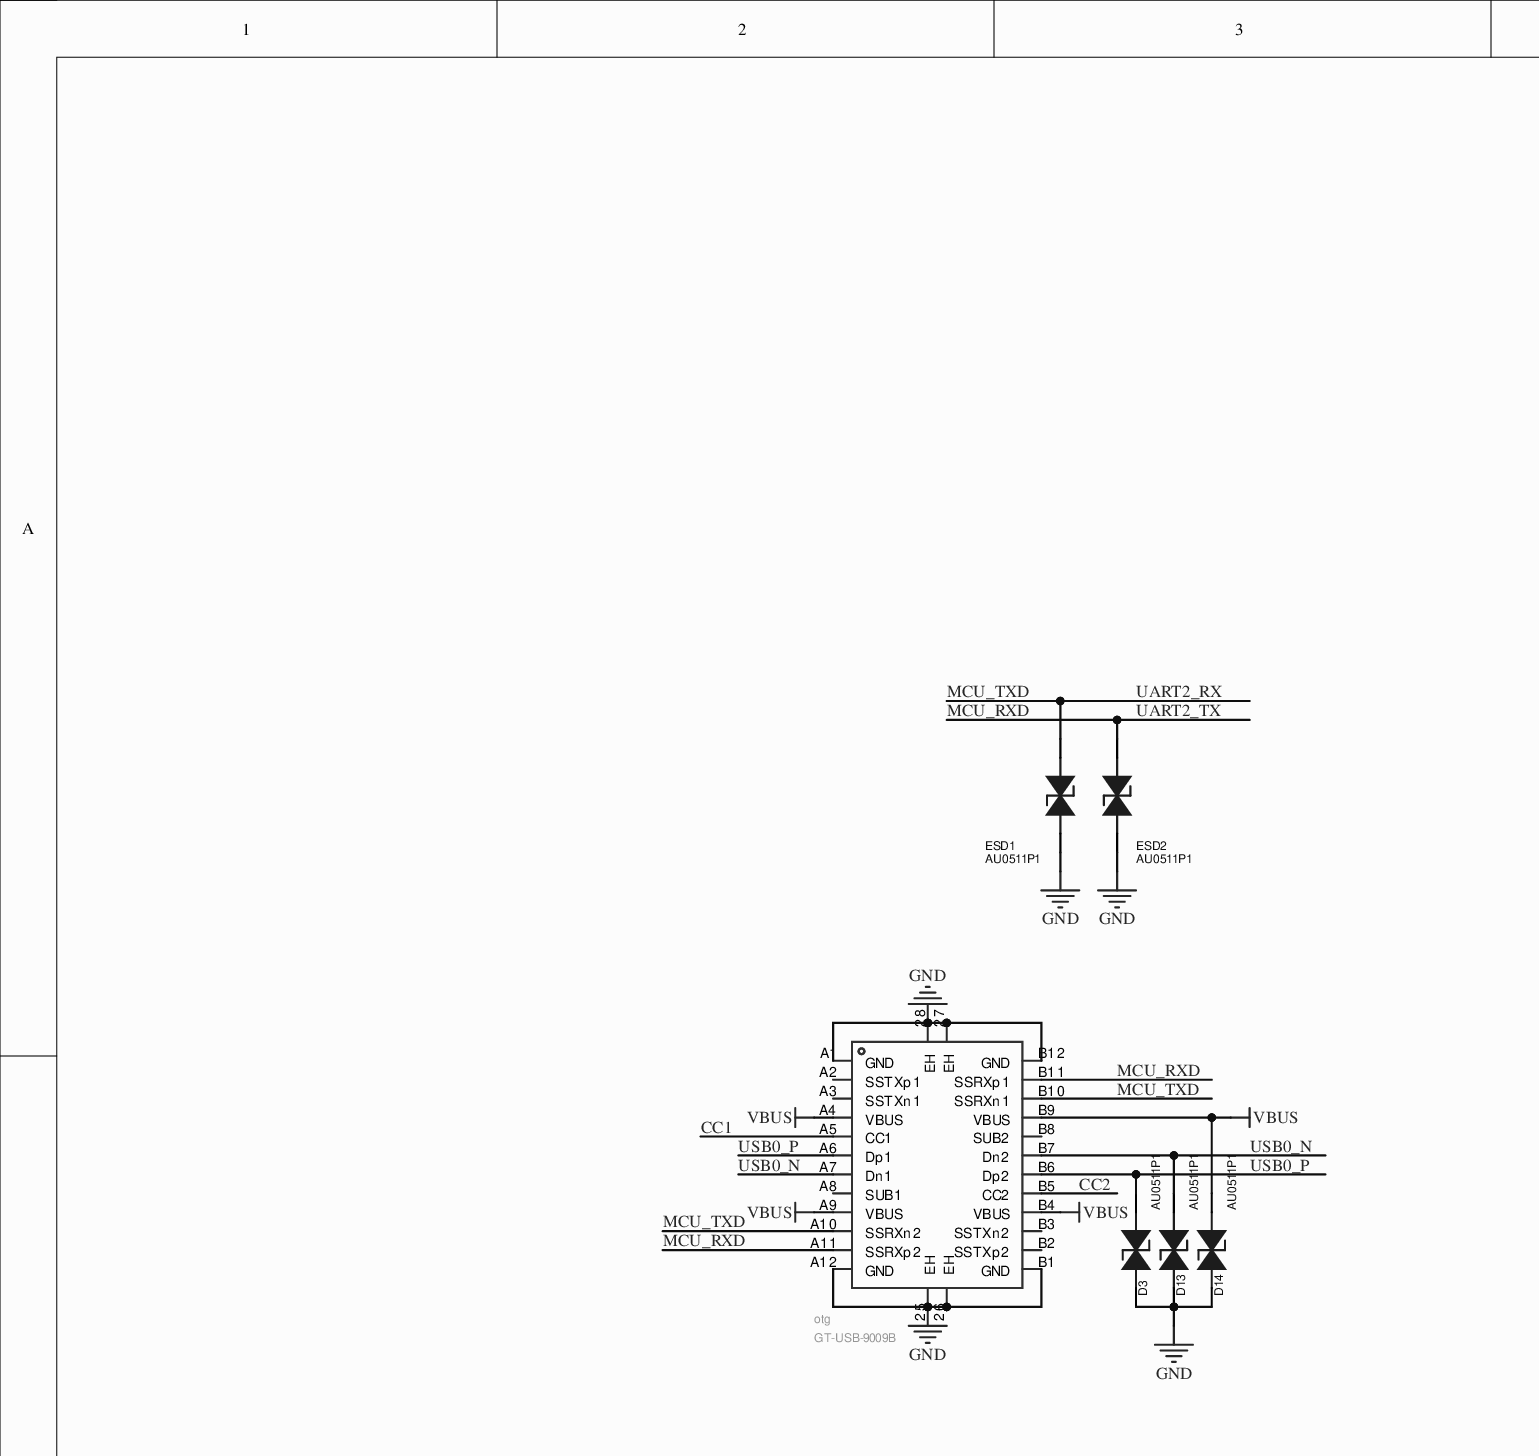
[diagram p0: MISC105407.SchDoc, top column 1 of 4]
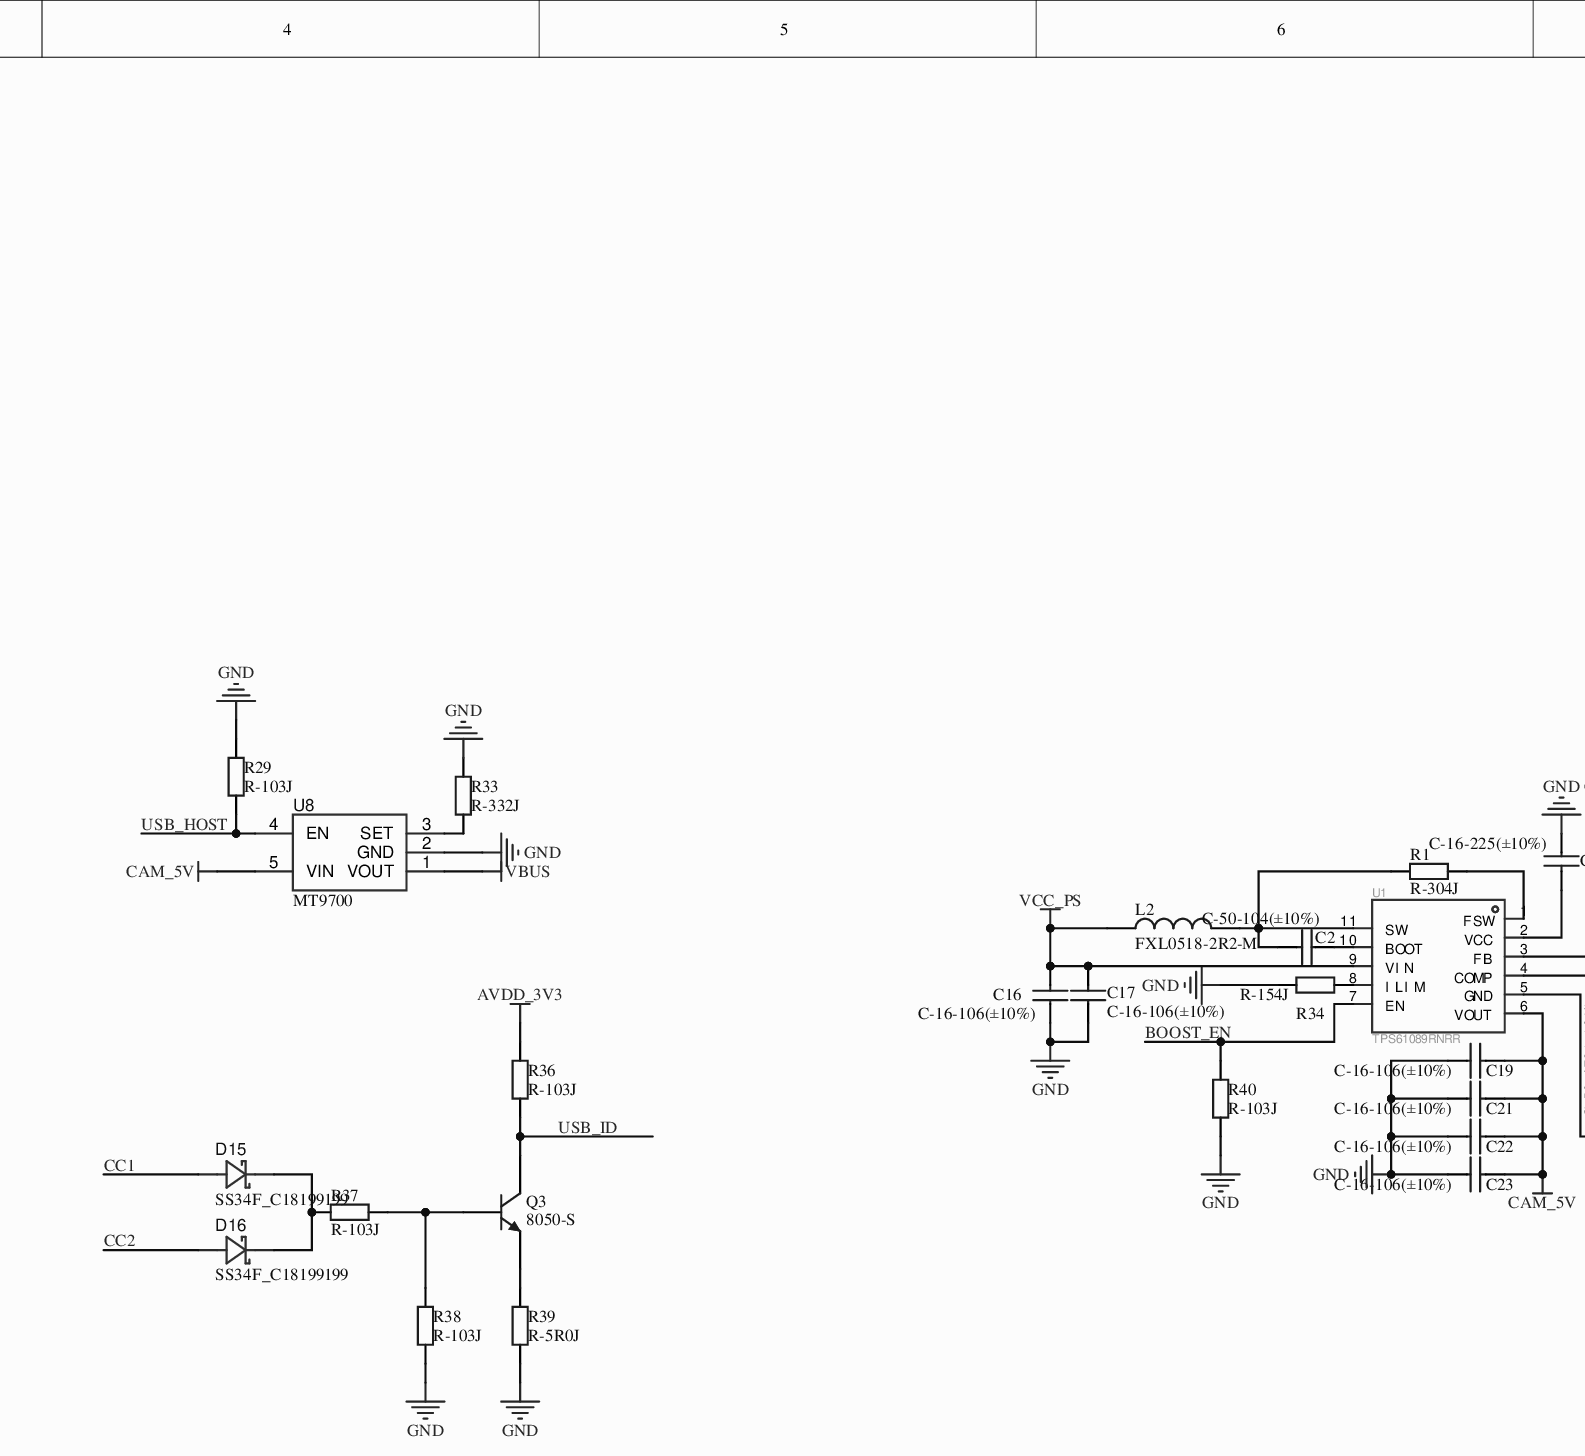
[diagram p1: MISC105407.SchDoc, top column 2 of 4]
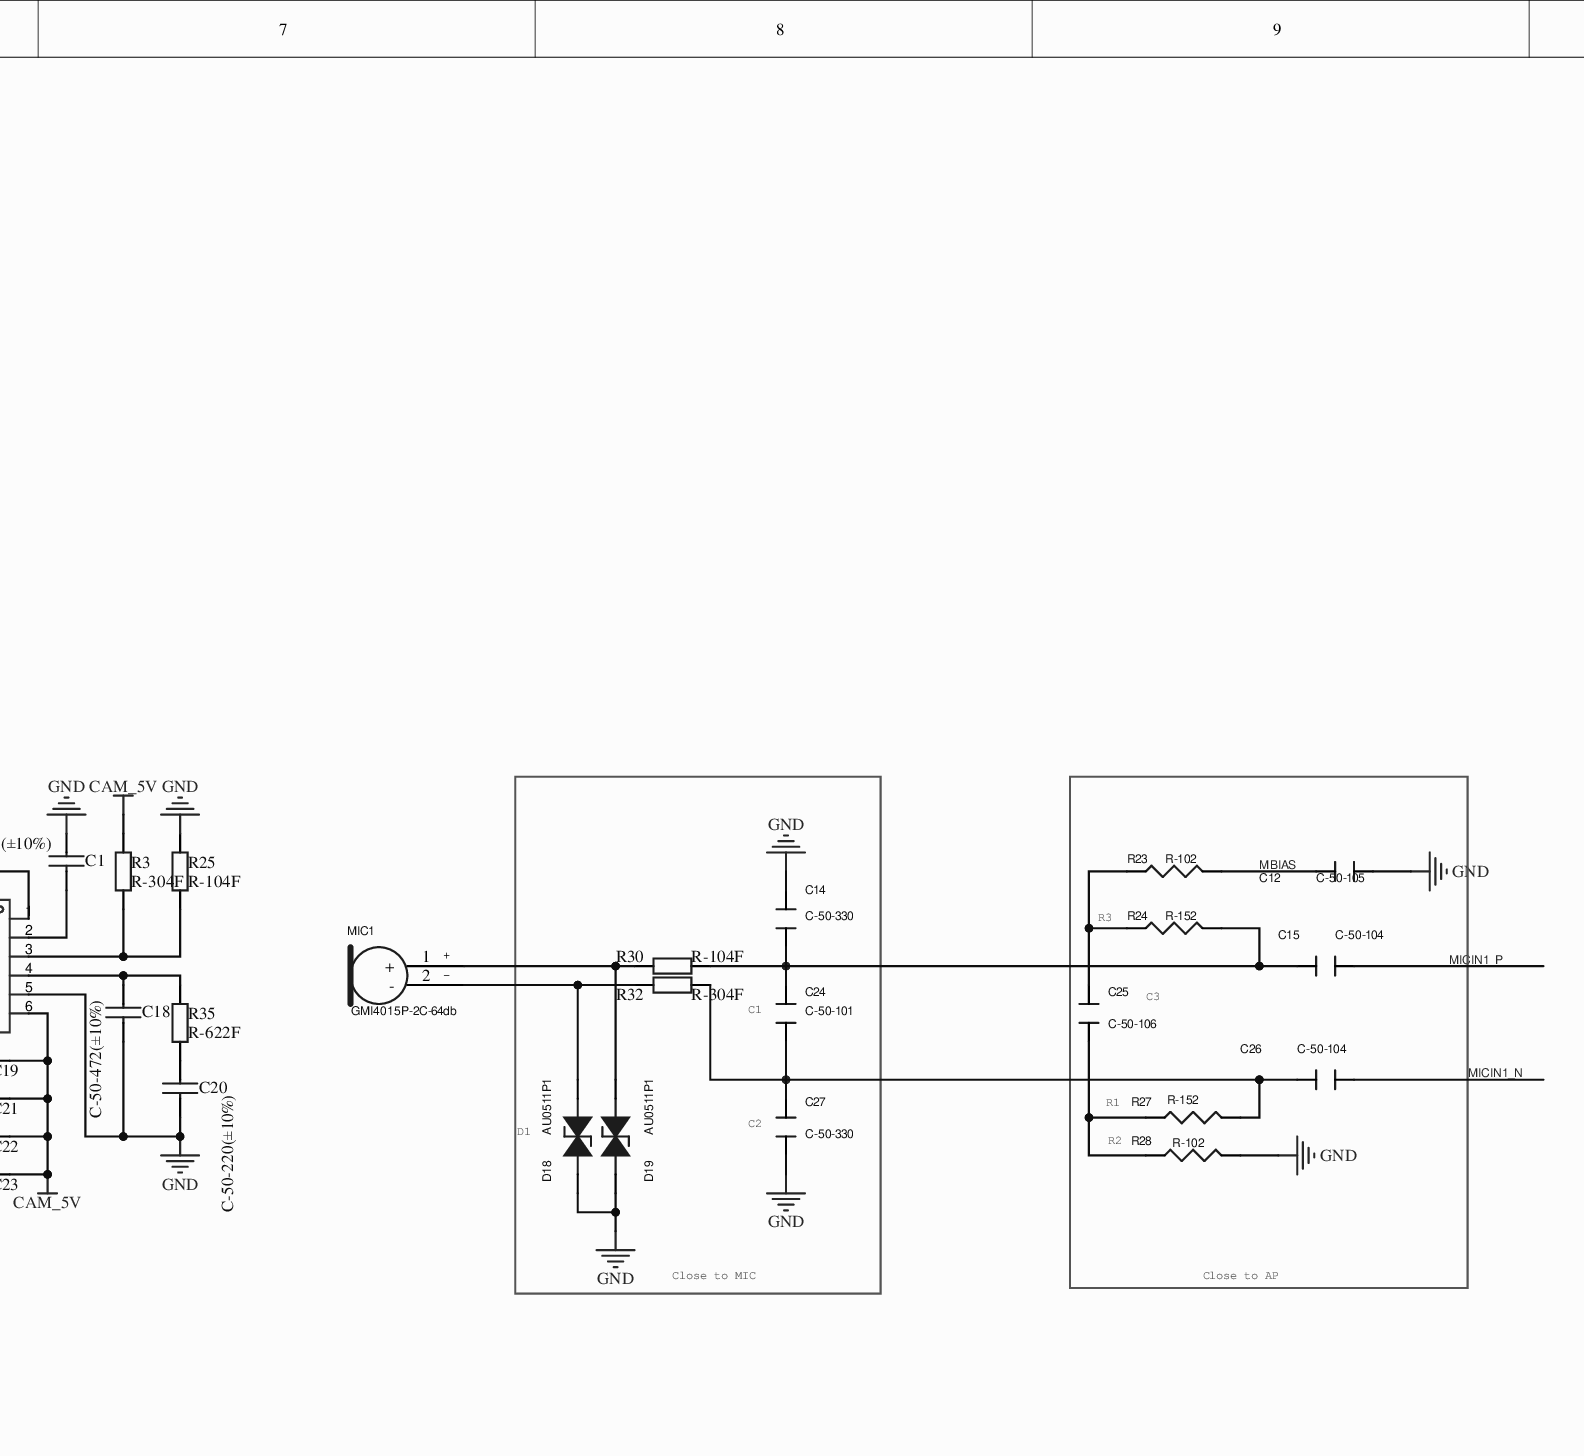
[diagram p2: MISC105407.SchDoc, top column 3 of 4]
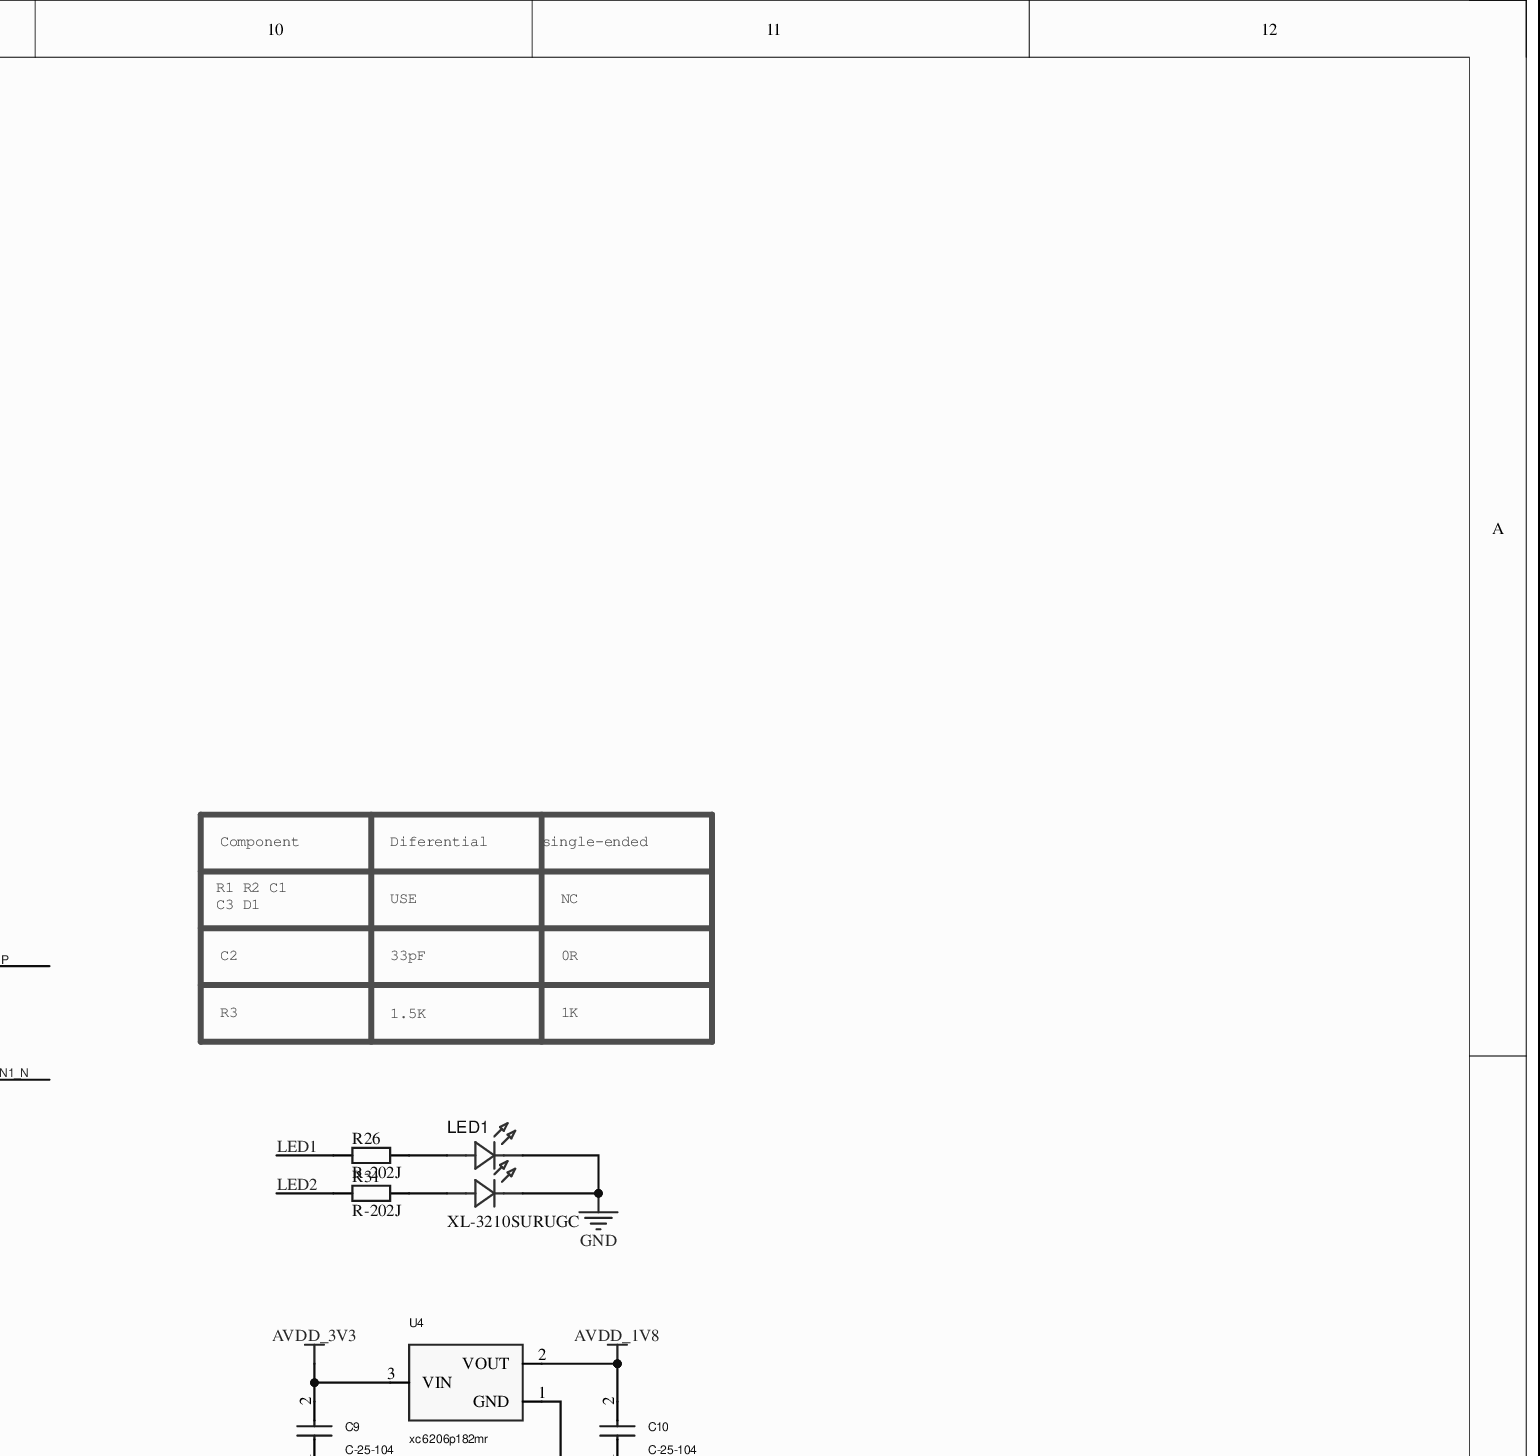
[diagram p3: MISC105407.SchDoc, top column 4 of 4]
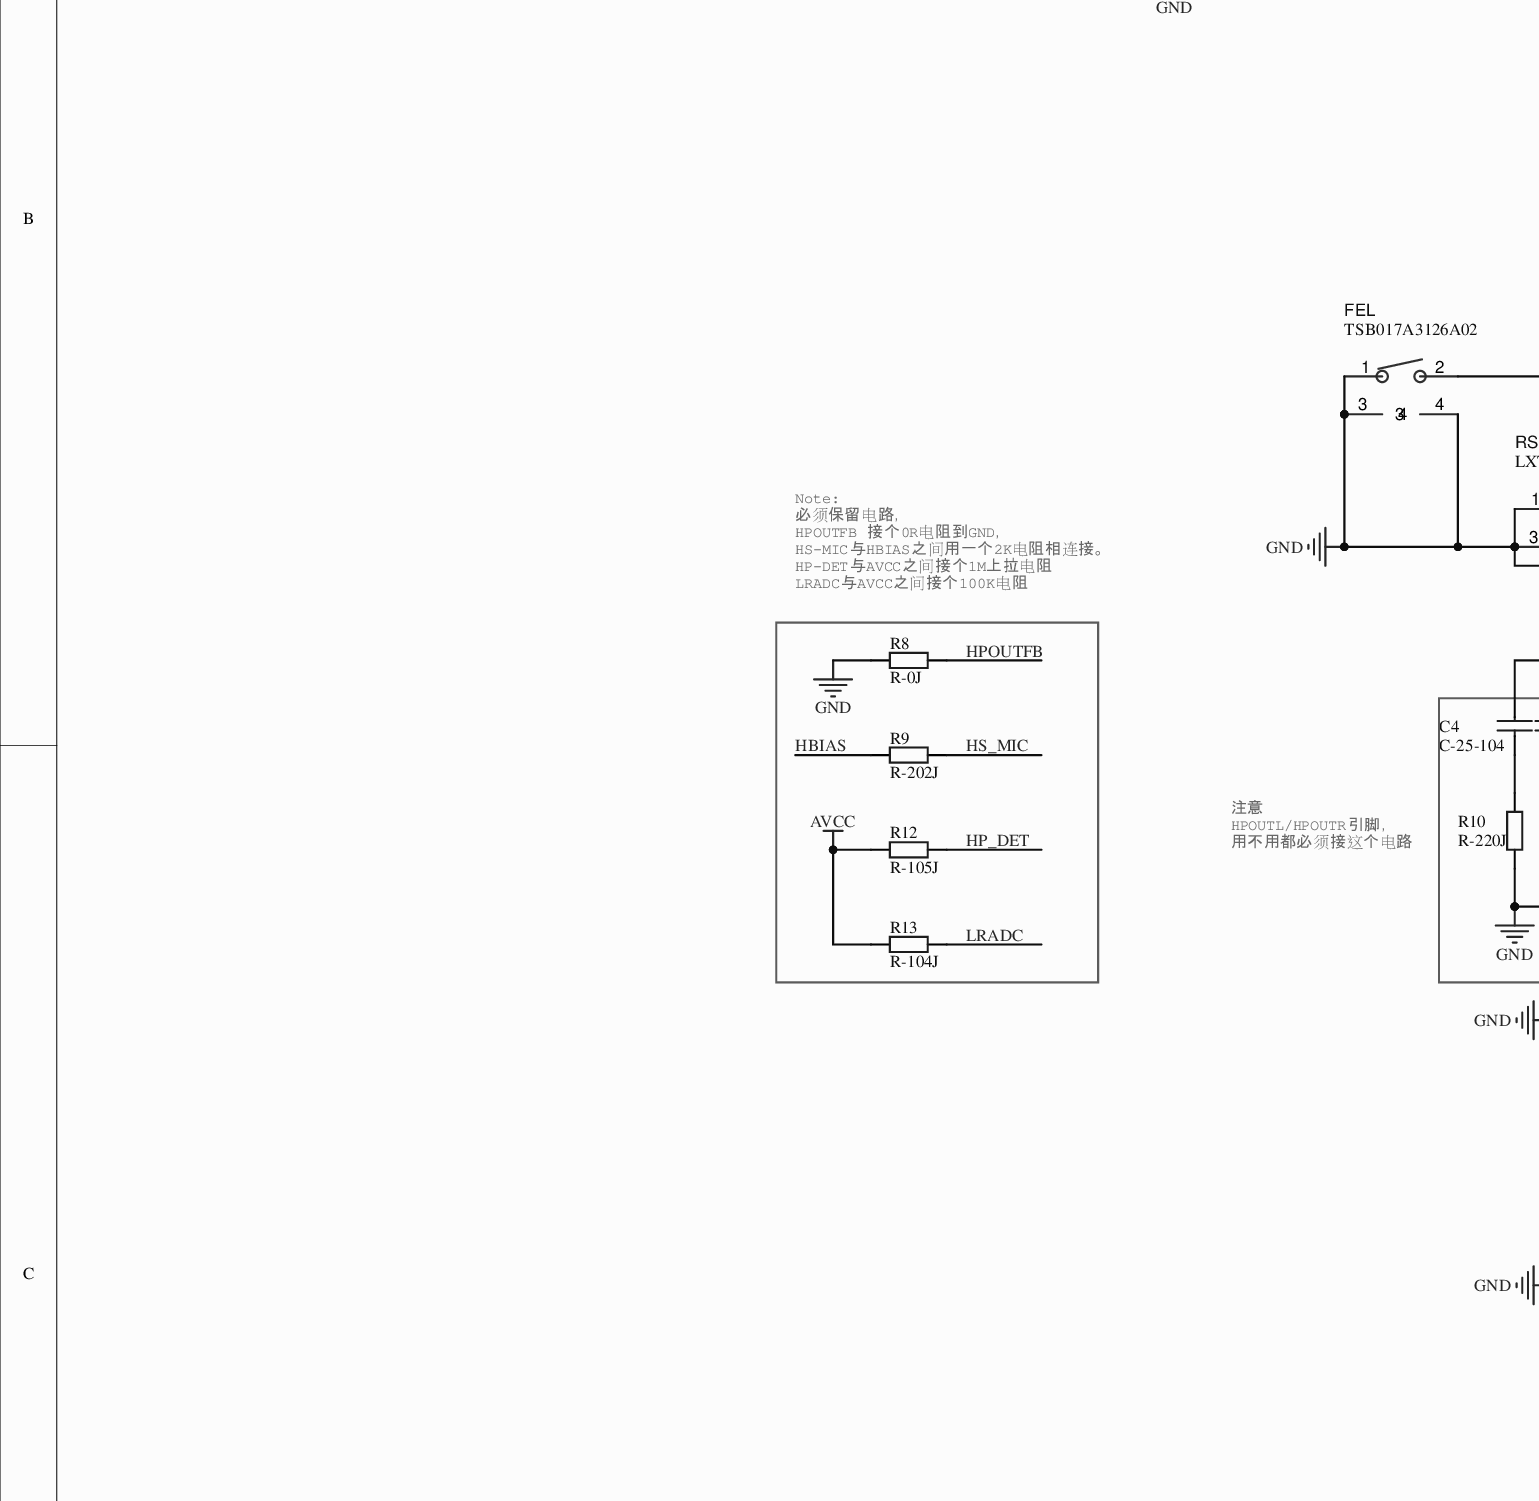
[diagram p4: MISC105407.SchDoc, centre column 1 of 4]
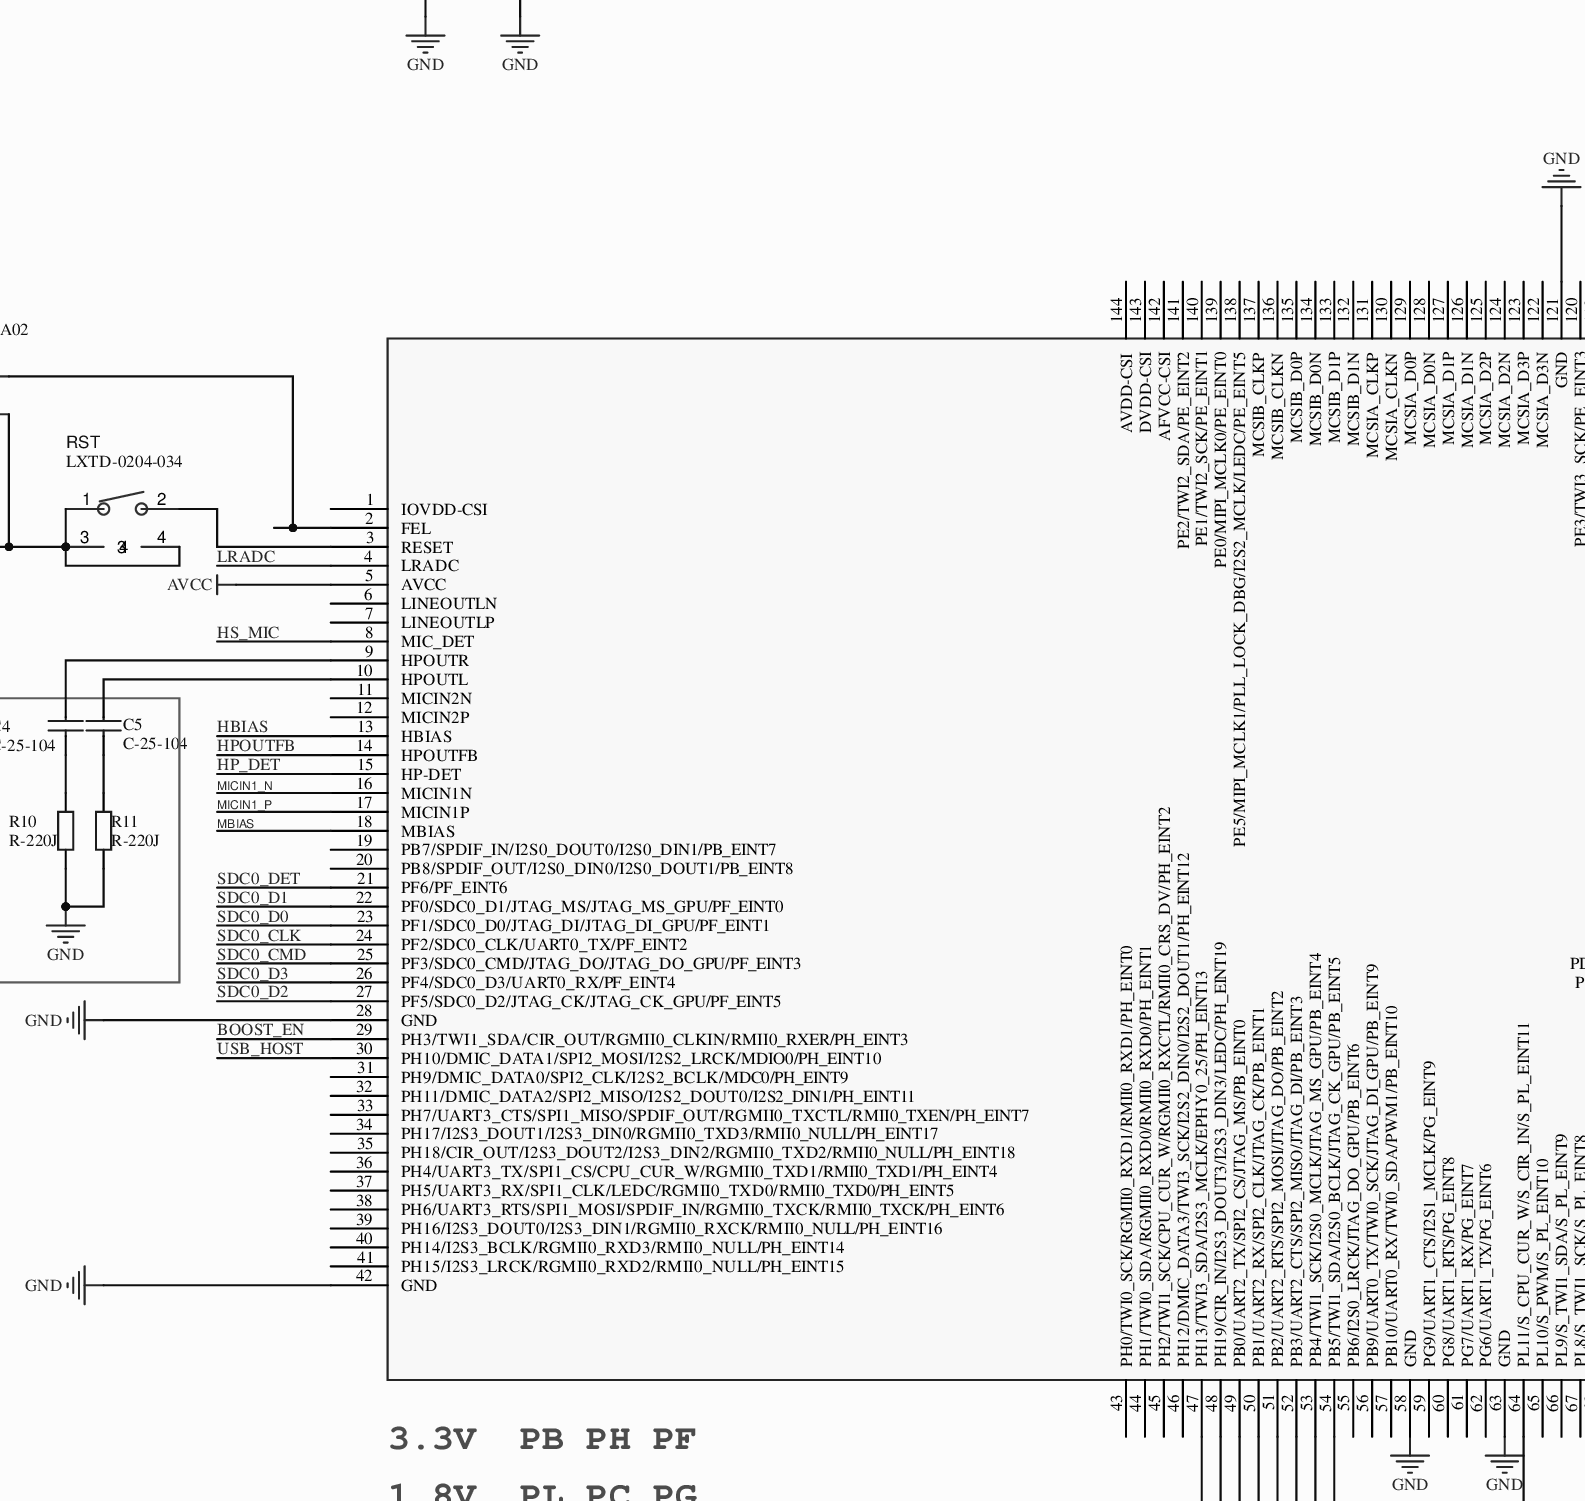
[diagram p5: MISC105407.SchDoc, centre column 2 of 4]
# Altium project MISC105407.PrjPcb (part 1 of 3)
1 sheet, 129 parts. Net scope: global (net labels, ports and power ports of the same name join across sheets).